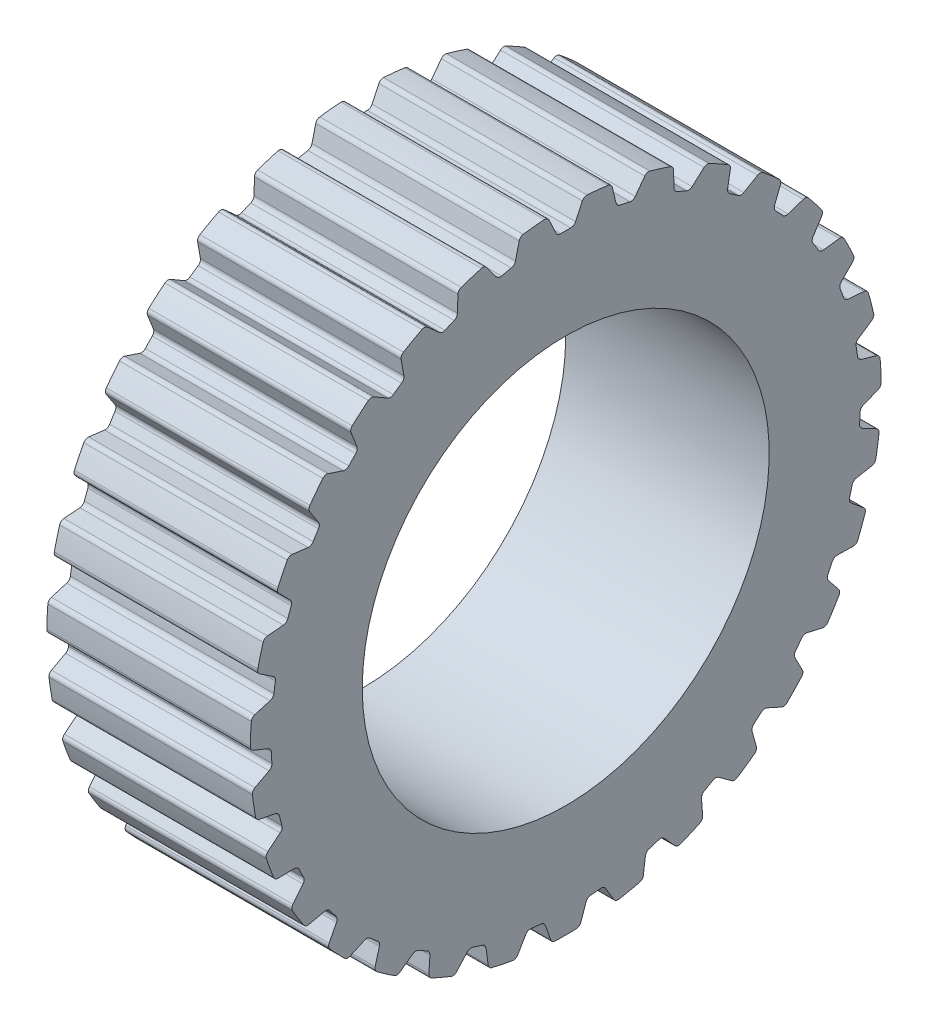
from build123d import *

# Parameters (mm, degrees)
CUT_EXTRUDE_2_REACH      = 41.998
PATTERN_CIRCULAR_3_COUNT = 31
CUT_EXTRUDE_3_DEPTH      = 40.995475706
CUT_EXTRUDE_3_DEPTH_BACK = 40.995475706
SKETCH_7_R               = 16


with BuildPart() as part:
    # 草图1 → 旋转1 (revolve)
    with BuildSketch(Plane.XY, mode=Mode.PRIVATE) as revolve_1_sk:
        Polygon((0, 11.5922), (0, 24.811), (16, 24.811), (16, 13), (19.2, 13), (19.2, 11.5922), align=None)
    revolve(revolve_1_sk.sketch.rotate(Axis((0, 0, 0), (1, 0, 0)), 90), axis=Axis((0, 0, 0), (1, 0, 0)))

    # 草图6 → 切除-拉伸2 (cut, up to next)
    with BuildSketch(Plane(origin=(0, 0, 0), x_dir=(0, 0, -1), z_dir=(1, 0, 0)), mode=Mode.PRIVATE) as cut_extrude_2_sk1:
        with BuildLine():
            Line((1.305475825, 24.535821724), (0.773177927, 23.394305198))
            ThreePointArc((0.773177927, 23.394305198), (0.618930764, 23.219924049), (0.394606345, 23.157638196))
            ThreePointArc((0.394606345, 23.157638196), (0, 23.161), (-0.394606345, 23.157638196))
            ThreePointArc((-0.394606345, 23.157638196), (-0.618930764, 23.219924049), (-0.773177927, 23.394305198))
            Line((-0.773177927, 23.394305198), (-1.305475825, 24.535821724))
            ThreePointArc((-1.305475825, 24.535821724), (-1.456643287, 24.702430638), (-1.67553492, 24.754359287))
            ThreePointArc((-1.67553492, 24.754359287), (-1.865052041, 24.740802369), (-2.054459788, 24.725794547))
            Line((-2.054459788, 24.725794547), (-2.669933516, 26.045682215))
            ThreePointArc((-2.669933516, 26.045682215), (0, 26.182171549), (2.669933516, 26.045682215))
            Line((2.669933516, 26.045682215), (2.054459788, 24.725794547))
            ThreePointArc((2.054459788, 24.725794547), (1.865052041, 24.740802369), (1.67553492, 24.754359287))
            ThreePointArc((1.67553492, 24.754359287), (1.456643287, 24.702430638), (1.305475825, 24.535821724))
        make_face()
    cut_extrude_2_tool1 = extrude(cut_extrude_2_sk1.sketch, amount=CUT_EXTRUDE_2_REACH, mode=Mode.PRIVATE) & part.part
    cut_extrude_2 = cut_extrude_2_tool1.solids().sort_by_distance((0, 25.005214, 0))[0]
    add(cut_extrude_2, mode=Mode.SUBTRACT)

    # 阵列(圆周)3: 切除-拉伸2 ×31 about axis
    pattern_circular_3_axis = Axis((0, 0, 0), (1, 0, 0))
    for i in range(1, PATTERN_CIRCULAR_3_COUNT):
        add(cut_extrude_2.rotate(pattern_circular_3_axis, i * 360 / PATTERN_CIRCULAR_3_COUNT), mode=Mode.SUBTRACT)

    # 草图7 → 切除-拉伸3 (cut, two sides: drawn at the far end of the back side and taken through both)
    with BuildSketch(Plane.ZY.offset(-CUT_EXTRUDE_3_DEPTH_BACK)):
        Circle(SKETCH_7_R)
    extrude(amount=CUT_EXTRUDE_3_DEPTH + CUT_EXTRUDE_3_DEPTH_BACK, mode=Mode.SUBTRACT)


solid = part.part
